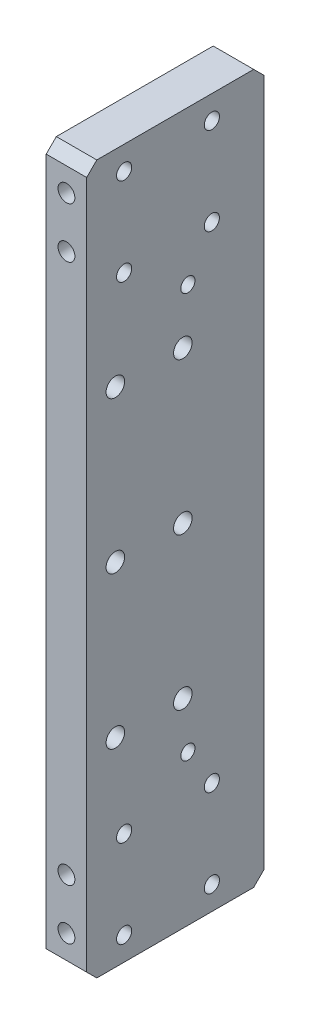
from build123d import *

# Parameters (mm, degrees)
SKETCH_1_W                                         = 68
SKETCH_1_H                                         = 190
BOSS_EXTRUDE_1_DEPTH                               = 12
SKETCH_9_W                                         = 68
SKETCH_9_H                                         = 10
BOSS_EXTRUDE_2_DEPTH                               = 12
F_4_5_4_5_HOLE_1_D                                 = 4.5
LINEAR_PATTERN_2_COUNT                             = 2
LINEAR_PATTERN_2_PITCH                             = 26
LINEAR_PATTERN_2_COUNT_DIR2                        = 2
LINEAR_PATTERN_2_PITCH_DIR2                        = 26
M5_SOCKET_HEAD_CAP_SCREW_COUNTERBORE_1_D           = 5.5
M5_SOCKET_HEAD_CAP_SCREW_COUNTERBORE_1_CBORE_D     = 10
M5_SOCKET_HEAD_CAP_SCREW_COUNTERBORE_1_CBORE_DEPTH = 5
LINEAR_PATTERN_3_COUNT                             = 3
LINEAR_PATTERN_3_PITCH                             = 45
LINEAR_PATTERN_3_COUNT_DIR2                        = 2
LINEAR_PATTERN_3_PITCH_DIR2                        = 20
SKETCH_14_W                                        = 20
SKETCH_14_H                                        = 215
CUT_EXTRUDE_4_DEPTH                                = 112.018016556
LINEAR_PATTERN_4_COUNT                             = 2
LINEAR_PATTERN_4_PITCH                             = 170
LINEAR_PATTERN_4_COPY_1_D                          = 4.5
LINEAR_PATTERN_4_COPY_2_D                          = 4.5
LINEAR_PATTERN_4_COPY_3_D                          = 4.5
M5_TAPPED_HOLE_1_D                                 = 4.2
LINEAR_PATTERN_5_COUNT                             = 2
LINEAR_PATTERN_5_PITCH                             = 120
LINEAR_PATTERN_6_COUNT                             = 2
LINEAR_PATTERN_6_PITCH                             = 15
CHAMFER_1_SIZE                                     = 3


with BuildPart() as part:
    # Sketch 1 → Boss-Extrude 1 (new body)
    with BuildSketch(Plane(origin=(0, 0, 0), x_dir=(0, 0, -1), z_dir=(1, 0, 0))):
        Rectangle(SKETCH_1_W, SKETCH_1_H)
    extrude(amount=BOSS_EXTRUDE_1_DEPTH)

    # Sketch 9 → Boss-Extrude 2 (add)
    with BuildSketch(Plane.ZY):
        with Locations((0, 100)):
            Rectangle(SKETCH_9_W, SKETCH_9_H)
        with Locations((0, -100)):
            Rectangle(SKETCH_9_W, SKETCH_9_H)
    extrude(amount=-BOSS_EXTRUDE_2_DEPTH)

    # Ø4.5 (4.5) Hole 1 (through all)
    with Locations(Plane.ZY):
        with Locations((22.9, -98)):
            f_4_5_4_5_hole_1 = Hole(F_4_5_4_5_HOLE_1_D / 2)

    # Linear Pattern 2: 4.5 _4.5_ Hole 1 2 × 2
    with Locations(*[(0, i * LINEAR_PATTERN_2_PITCH, -j * LINEAR_PATTERN_2_PITCH_DIR2) for i in range(LINEAR_PATTERN_2_COUNT) for j in range(LINEAR_PATTERN_2_COUNT_DIR2) if (i, j) != (0, 0)]):
        add(f_4_5_4_5_hole_1, mode=Mode.SUBTRACT)

    # M5 Socket Head Cap Screw Counterbore 1 (through all)
    with Locations(Plane.ZY):
        with Locations((5.5, 44)):
            m5_socket_head_cap_screw_counterbore_1 = CounterBoreHole(M5_SOCKET_HEAD_CAP_SCREW_COUNTERBORE_1_D / 2, M5_SOCKET_HEAD_CAP_SCREW_COUNTERBORE_1_CBORE_D / 2, M5_SOCKET_HEAD_CAP_SCREW_COUNTERBORE_1_CBORE_DEPTH)

    # Linear Pattern 3: M5 Socket Head Cap Screw Counterbore 1 3 × 2
    with Locations(*[(0, -i * LINEAR_PATTERN_3_PITCH, j * LINEAR_PATTERN_3_PITCH_DIR2) for i in range(LINEAR_PATTERN_3_COUNT) for j in range(LINEAR_PATTERN_3_COUNT_DIR2) if (i, j) != (0, 0)]):
        add(m5_socket_head_cap_screw_counterbore_1, mode=Mode.SUBTRACT)

    # Sketch 14 → Cut-Extrude 4 (cut, through all)
    with BuildSketch(Plane.ZY):
        with Locations((-28.5, -2.5)):
            Rectangle(SKETCH_14_W, SKETCH_14_H)
    extrude(amount=-CUT_EXTRUDE_4_DEPTH, mode=Mode.SUBTRACT)

    # Linear Pattern 4: Ø4.5 (4.5) Hole 1 ×2
    with Locations(*[(0, i * LINEAR_PATTERN_4_PITCH, 0) for i in range(1, LINEAR_PATTERN_4_COUNT)]):
        add(f_4_5_4_5_hole_1, mode=Mode.SUBTRACT)

    # Linear Pattern 4 copy 1 (through all)
    with Locations(Plane(origin=(0, 170, -26), x_dir=(0, 0, 1), z_dir=(-1, 0, 0))):
        with Locations((22.9, -98)):
            Hole(LINEAR_PATTERN_4_COPY_1_D / 2)

    # Linear Pattern 4 copy 2 (through all)
    with Locations(Plane(origin=(0, 196, 0), x_dir=(0, 0, 1), z_dir=(-1, 0, 0))):
        with Locations((22.9, -98)):
            Hole(LINEAR_PATTERN_4_COPY_2_D / 2)

    # Linear Pattern 4 copy 3 (through all)
    with Locations(Plane(origin=(0, 196, -26), x_dir=(0, 0, 1), z_dir=(-1, 0, 0))):
        with Locations((22.9, -98)):
            Hole(LINEAR_PATTERN_4_COPY_3_D / 2)

    # M5 Tapped Hole 1 (through all)
    with Locations(Plane.ZY):
        with Locations((4, 59.5)):
            m5_tapped_hole_1 = Hole(M5_TAPPED_HOLE_1_D / 2)

    # Linear Pattern 5: M5 Tapped Hole 1 ×2
    with Locations(*[(0, -i * LINEAR_PATTERN_5_PITCH, 0) for i in range(1, LINEAR_PATTERN_5_COUNT)]):
        add(m5_tapped_hole_1, mode=Mode.SUBTRACT)

    # Sketch 17 → M6 Tapped Hole 1 (revolve, cut)
    with BuildSketch(Plane(origin=(6, 95, 34), x_dir=(0, -1, 0), z_dir=(1, 0, 0))):
        Polygon((0, 0), (0, 16.502151548), (2.5, 15), (2.5, 0), align=None)
    m6_tapped_hole_1 = revolve(axis=Axis((6, 95, 40.35), (0, 0, -1)), mode=Mode.SUBTRACT)

    # Linear Pattern 6: M6 Tapped Hole 1 ×2
    with Locations(*[(0, -i * LINEAR_PATTERN_6_PITCH, 0) for i in range(1, LINEAR_PATTERN_6_COUNT)]):
        add(m6_tapped_hole_1, mode=Mode.SUBTRACT)

    # Mirror 1: M6 Tapped Hole 1 across plane
    add(m6_tapped_hole_1.mirror(Plane.ZX), mode=Mode.SUBTRACT)

    # Mirror 1 copy 1 sketch → Mirror 1 copy 1 (revolve, cut)
    with BuildSketch(Plane(origin=(6, -80, 34), x_dir=(0, 1, 0), z_dir=(1, 0, 0))):
        Polygon((0, 0), (0, -16.502151548), (2.5, -15), (2.5, 0), align=None)
    revolve(axis=Axis((6, -80, 40.35), (0, 0, 1)), mode=Mode.SUBTRACT)

    # Chamfer 1
    chamfer_1_edges = [part.edges().sort_by_distance(p)[0] for p in [
        (6, 105, 34),
        (6, -105, 34),
        (6, -105, -18.5),
        (6, 105, -18.5),
    ]]
    chamfer(chamfer_1_edges, length=CHAMFER_1_SIZE)


solid = part.part
